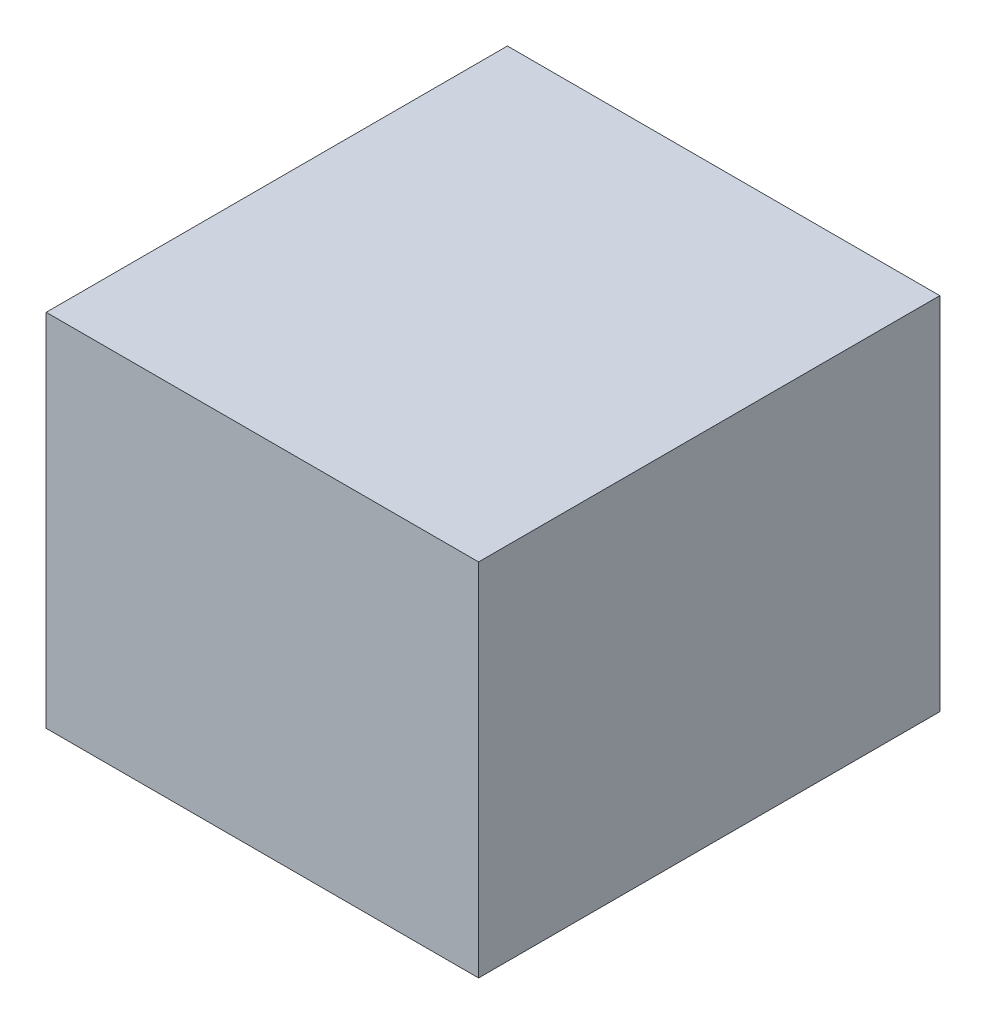
SolidWorks part; units mm, degrees
ref_plane "Front Plane" through (0, 0, 0) normal (0, 0, 1) x (1, 0, 0)
ref_plane "Top Plane" through (0, 0, 0) normal (0, 1, 0) x (1, 0, 0)
ref_plane "Right Plane" through (0, 0, 0) normal (1, 0, 0) x (0, 0, -1)
other "Configuration Table"
sketch "Sketch1" plane through (0, 0, 0) normal (0, 1, 0) x (1, 0, 0)
  line L1 (-150, 160) -> (150, 160)
  line L2 (-150, 160) -> (-150, -160)
  line L3 (-150, -160) -> (150, -160)
  line L4 (150, 160) -> (150, -160)
  line L5 (-150, 160) -> (150, -160) construction
  line L6 (-150, -160) -> (150, 160) construction
  point P0 (0, 0)
  dimension "D1" = 300
  dimension "D2" = 320
extrude "Boss-Extrude1" add sketch "Sketch1" along normal blind 250
